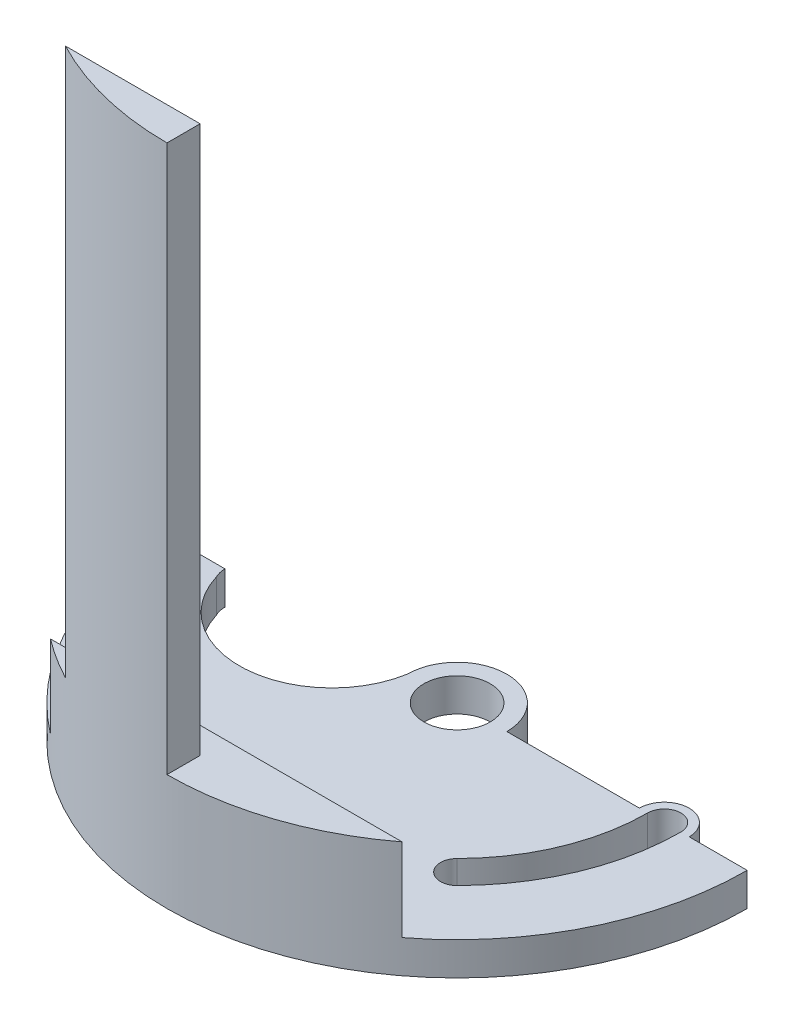
from build123d import *

# Parameters (mm, degrees)
SKETCH1_R                = 17.5
BOSS_EXTRUDE1_DEPTH      = 30
SKETCH2_R                = 4
BOSS_EXTRUDE2_DEPTH      = 2
CHAMFER1_SIZE            = 1
SKETCH4_R                = 2
BOSS_EXTRUDE3_DEPTH      = 12
SKETCH5_R                = 1.5
CUT_EXTRUDE1_DEPTH       = 12
CUT_EXTRUDE2_DEPTH       = 39.890872965
CUT_EXTRUDE2_DEPTH_BACK  = 39.890872965
SKETCH6_W                = 34.294260261
SKETCH6_H                = 28
CUT_EXTRUDE3_DEPTH       = 39.890872965
CUT_EXTRUDE3_DEPTH_BACK  = 39.890872965
SKETCH7_W                = 3
SKETCH7_H                = 23
CUT_EXTRUDE4_DEPTH       = 39.890872965
CUT_EXTRUDE4_DEPTH_BACK  = 39.890872965
SKETCH8_W                = 1.5
SKETCH8_H                = 5
CUT_EXTRUDE5_DEPTH       = 48.908767465
CUT_EXTRUDE5_DEPTH_BACK  = 48.908767465
SKETCH9_W                = 8.124038405
SKETCH9_H                = 23
CUT_EXTRUDE6_DEPTH       = 51.482670294
CUT_EXTRUDE6_DEPTH_BACK  = 0.5
SKETCH10_R               = 0.641252557
SKETCH11_R               = 17.5
BOSS_EXTRUDE4_DEPTH      = 5
CUT_EXTRUDE8_DEPTH       = 4
CUT_EXTRUDE9_DEPTH       = 39.890872965
CUT_EXTRUDE9_DEPTH_BACK  = 39.890872965
SKETCH13_W               = 19.268240878
SKETCH13_H               = 2
SKETCH14_R               = 2
CUT_EXTRUDE10_DEPTH      = 6
CUT_EXTRUDE11_DEPTH      = 39.890872965
CUT_EXTRUDE11_DEPTH_BACK = 39.890872965
SKETCH16_W               = 3.25
SKETCH16_H               = 3
CUT_EXTRUDE12_DEPTH      = 36.178118199
CUT_EXTRUDE13_START      = -17
SKETCH18_R               = 17.5
CUT_EXTRUDE13_DEPTH      = 17
BOSS_EXTRUDE5_DEPTH      = 3
BOSS_EXTRUDE6_DEPTH      = 13
CUT_EXTRUDE14_DEPTH      = 46.348649373
CUT_EXTRUDE14_DEPTH_BACK = 46.348649373
SKETCH21_R               = 1.5
SKETCH22_R               = 1
BOSS_EXTRUDE7_DEPTH      = 5
CUT_EXTRUDE15_DEPTH      = 5


with BuildPart() as part:
    # Sketch1 → Boss-Extrude1 (new body)
    with BuildSketch(Plane(origin=(0, 0, 0), x_dir=(1, 0, 0), z_dir=(0, 1, 0))):
        with Locations(Location((0, 0, 0), (0, 0, 270))):
            Circle(SKETCH1_R)
    extrude(amount=BOSS_EXTRUDE1_DEPTH)

    # Sketch2 → Boss-Extrude2 (add)
    with BuildSketch(Plane.XZ):
        with Locations(Location((0, 0, 0), (0, 0, 270))):
            Circle(SKETCH2_R)
    extrude(amount=BOSS_EXTRUDE2_DEPTH)

    # Chamfer1
    chamfer1_edges = [part.edges().sort_by_distance(p)[0] for p in [
        (0, 0, 4),
    ]]
    chamfer(chamfer1_edges, length=CHAMFER1_SIZE)

    # Sketch4 → Boss-Extrude3 (add)
    with BuildSketch(Plane.XZ.offset(2)):
        with Locations(Location((0, 0, 0), (0, 0, 270))):
            Circle(SKETCH4_R)
    extrude(amount=BOSS_EXTRUDE3_DEPTH)

    # Sketch5 → Cut-Extrude1 (cut)
    with BuildSketch(Plane.XZ.offset(14)):
        with Locations(Location((0, 0, 0), (0, 0, 270))):
            Circle(SKETCH5_R)
    extrude(amount=-CUT_EXTRUDE1_DEPTH, mode=Mode.SUBTRACT)

    # Sketch6 → Cut-Extrude2 (cut, two sides: drawn at the far end of the back side and taken through both)
    with BuildSketch(Plane(origin=(0, 0, 0), x_dir=(0, 0, -1), z_dir=(1, 0, 0)).offset(-CUT_EXTRUDE2_DEPTH_BACK)):
        with Locations((4.647130131, 16)):
            Rectangle(SKETCH6_W, SKETCH6_H)
    extrude(amount=CUT_EXTRUDE2_DEPTH + CUT_EXTRUDE2_DEPTH_BACK, mode=Mode.SUBTRACT)

    # Sketch7 → Cut-Extrude3 (cut, two sides: drawn at the far end of the back side and taken through both)
    with BuildSketch(Plane(origin=(0, 0, 0), x_dir=(0, 0, -1), z_dir=(1, 0, 0)).offset(-CUT_EXTRUDE3_DEPTH_BACK)):
        with Locations((-14, 18.5)):
            Rectangle(SKETCH7_W, SKETCH7_H)
    extrude(amount=CUT_EXTRUDE3_DEPTH + CUT_EXTRUDE3_DEPTH_BACK, mode=Mode.SUBTRACT)

    # Sketch8 → Cut-Extrude4 (cut, two sides: drawn at the far end of the back side and taken through both)
    with BuildSketch(Plane(origin=(0, 0, 0), x_dir=(0, 0, -1), z_dir=(1, 0, 0)).offset(-CUT_EXTRUDE4_DEPTH_BACK)):
        with Locations((-13.25, 4.5)):
            Rectangle(SKETCH8_W, SKETCH8_H)
    extrude(amount=CUT_EXTRUDE4_DEPTH + CUT_EXTRUDE4_DEPTH_BACK, mode=Mode.SUBTRACT)

    # Sketch9 → Cut-Extrude5 (cut, two sides: drawn at the far end of the back side and taken through both)
    with BuildSketch(Plane(origin=(0, 0, 15.5), x_dir=(-1, 0, 0), z_dir=(0, 0, -1)).offset(-CUT_EXTRUDE5_DEPTH_BACK)):
        with Locations((-4.062019203, 18.5)):
            Rectangle(SKETCH9_W, SKETCH9_H)
    extrude(amount=CUT_EXTRUDE5_DEPTH + CUT_EXTRUDE5_DEPTH_BACK, mode=Mode.SUBTRACT)

    # Sketch10 → Cut-Extrude6 (cut, two sides: drawn at the far end of the back side and taken through both)
    with BuildSketch(Plane(origin=(0, 30, 0), x_dir=(1, 0, 0), z_dir=(0, 1, 0)).offset(-CUT_EXTRUDE6_DEPTH_BACK)):
        with Locations(Location((-1.034007802, -16.523277445, 0), (0, 0, 270))):
            Circle(SKETCH10_R)
    extrude(amount=CUT_EXTRUDE6_DEPTH + CUT_EXTRUDE6_DEPTH_BACK, mode=Mode.SUBTRACT)

    # Sketch11 → Boss-Extrude4 (add)
    with BuildSketch(Plane(origin=(0, 2, 0), x_dir=(1, 0, 0), z_dir=(0, 1, 0))):
        with Locations(Location((0, 0, 0), (0, 0, 270))):
            Circle(SKETCH11_R)
    extrude(amount=BOSS_EXTRUDE4_DEPTH)

    # Sketch12 → Cut-Extrude8 (cut)
    with BuildSketch(Plane(origin=(0, 7, 0), x_dir=(1, 0, 0), z_dir=(0, 1, 0))):
        with BuildLine():
            Line((-17.5, 0), (-3, 0))
            ThreePointArc((-3, 0), (0, 3), (3, 0))
            Line((3, 0), (11, 0))
            ThreePointArc((11, 0), (12.5, 1.5), (14, 0))
            Line((14, 0), (18.571441089, 0))
            Line((18.571441089, 0), (18.571441089, 21.35501059))
            Line((18.571441089, 21.35501059), (-17.5, 21.35501059))
            Line((-17.5, 21.35501059), (-17.5, 0))
        make_face()
    extrude(amount=-CUT_EXTRUDE8_DEPTH, mode=Mode.SUBTRACT)

    # Sketch13 → Cut-Extrude9 (cut, two sides: drawn at the far end of the back side and taken through both)
    with BuildSketch(Plane(origin=(0, 0, 0), x_dir=(0, 0, -1), z_dir=(1, 0, 0)).offset(-CUT_EXTRUDE9_DEPTH_BACK)):
        with Locations((-4.288358488, 6)):
            Rectangle(SKETCH13_W, SKETCH13_H)
    extrude(amount=CUT_EXTRUDE9_DEPTH + CUT_EXTRUDE9_DEPTH_BACK, mode=Mode.SUBTRACT)

    # Sketch14 → Cut-Extrude10 (cut)
    with BuildSketch(Plane(origin=(0, 5, 0), x_dir=(1, 0, 0), z_dir=(0, 1, 0))):
        with Locations(Location((0, 0, 0), (0, 0, 90))):
            Circle(SKETCH14_R)
    extrude(amount=-CUT_EXTRUDE10_DEPTH, mode=Mode.SUBTRACT)

    # Sketch16 → Cut-Extrude11 (cut, two sides: drawn at the far end of the back side and taken through both)
    with BuildSketch(Plane(origin=(0, 0, 0), x_dir=(0, 0, -1), z_dir=(1, 0, 0)).offset(-CUT_EXTRUDE11_DEPTH_BACK)):
        with Locations((15.875, 1.5)):
            Rectangle(SKETCH16_W, SKETCH16_H)
    extrude(amount=CUT_EXTRUDE11_DEPTH + CUT_EXTRUDE11_DEPTH_BACK, mode=Mode.SUBTRACT)

    # Sketch17 → Cut-Extrude12 (cut, through all)
    with BuildSketch(Plane(origin=(0, 5, 0), x_dir=(1, 0, 0), z_dir=(0, 1, 0))):
        with BuildLine():
            ThreePointArc((9.545941546, -9.545941546), (12.472373689, -5.166226337), (13.5, 0))
            ThreePointArc((13.5, 0), (12.5, 1), (11.5, 0))
            ThreePointArc((11.5, 0), (10.624614624, -4.400859472), (8.131727984, -8.131727984))
            ThreePointArc((8.131727984, -8.131727984), (8.131727984, -9.545941546), (9.545941546, -9.545941546))
        make_face()
    extrude(amount=-CUT_EXTRUDE12_DEPTH, mode=Mode.SUBTRACT)

    # Sketch18 → Cut-Extrude13 (cut)
    with BuildSketch(Plane(origin=(0, 3, 0), x_dir=(1, 0, 0), z_dir=(0, 1, 0)).offset(CUT_EXTRUDE13_START)):
        Circle(SKETCH18_R)
    extrude(amount=CUT_EXTRUDE13_DEPTH, mode=Mode.SUBTRACT)

    # Sketch19 → Boss-Extrude5 (add)
    with BuildSketch(Plane(origin=(0, 7, 0), x_dir=(1, 0, 0), z_dir=(0, 1, 0))):
        with BuildLine():
            Line((10.602574241, -13.922478927), (-10.602574241, -13.922478927))
            ThreePointArc((-10.602574241, -13.922478927), (-9.396470001, -14.763344862), (-8.124038405, -15.5))
            Line((-8.124038405, -15.5), (0, -15.5))
            Line((0, -15.5), (0, -17.5))
            ThreePointArc((0, -17.5), (5.594936049, -16.581516535), (10.602574241, -13.922478927))
        make_face()
    extrude(amount=BOSS_EXTRUDE5_DEPTH)

    # Sketch20 → Boss-Extrude6 (add)
    with BuildSketch(Plane(origin=(0, 30, 0), x_dir=(1, 0, 0), z_dir=(0, 1, 0))):
        with BuildLine():
            Line((0, -17.5), (0, -15.5))
            Line((0, -15.5), (-8.124038405, -15.5))
            ThreePointArc((-8.124038405, -15.5), (-4.183300133, -16.992645468), (0, -17.5))
        make_face()
    extrude(amount=BOSS_EXTRUDE6_DEPTH)

    # Sketch21 → Cut-Extrude14 (cut, two sides: drawn at the far end of the back side and taken through both)
    with BuildSketch(Plane(origin=(0, 5, 0), x_dir=(1, 0, 0), z_dir=(0, 1, 0)).offset(-CUT_EXTRUDE14_DEPTH_BACK)):
        with Locations((-12.5, 0)):
            Circle(SKETCH21_R)
    extrude(amount=CUT_EXTRUDE14_DEPTH + CUT_EXTRUDE14_DEPTH_BACK, mode=Mode.SUBTRACT)

    # Sketch22 → Boss-Extrude7 (add)
    with BuildSketch(Plane(origin=(0, 5, 0), x_dir=(1, 0, 0), z_dir=(0, 1, 0))):
        with Locations(Location((-10.580817493, -6.655546647, 0), (0, 0, 90))):
            Circle(SKETCH22_R)
    extrude(amount=BOSS_EXTRUDE7_DEPTH)

    # Sketch23 → Cut-Extrude15 (cut)
    with BuildSketch(Plane(origin=(0, 5, 0), x_dir=(1, 0, 0), z_dir=(0, 1, 0))):
        with BuildLine():
            Line((-14, 0), (-3, 0))
            ThreePointArc((-3, 0), (-8.5, -4.635701065), (-14, 0))
        make_face()
    extrude(amount=-CUT_EXTRUDE15_DEPTH, mode=Mode.SUBTRACT)


solid = part.part
